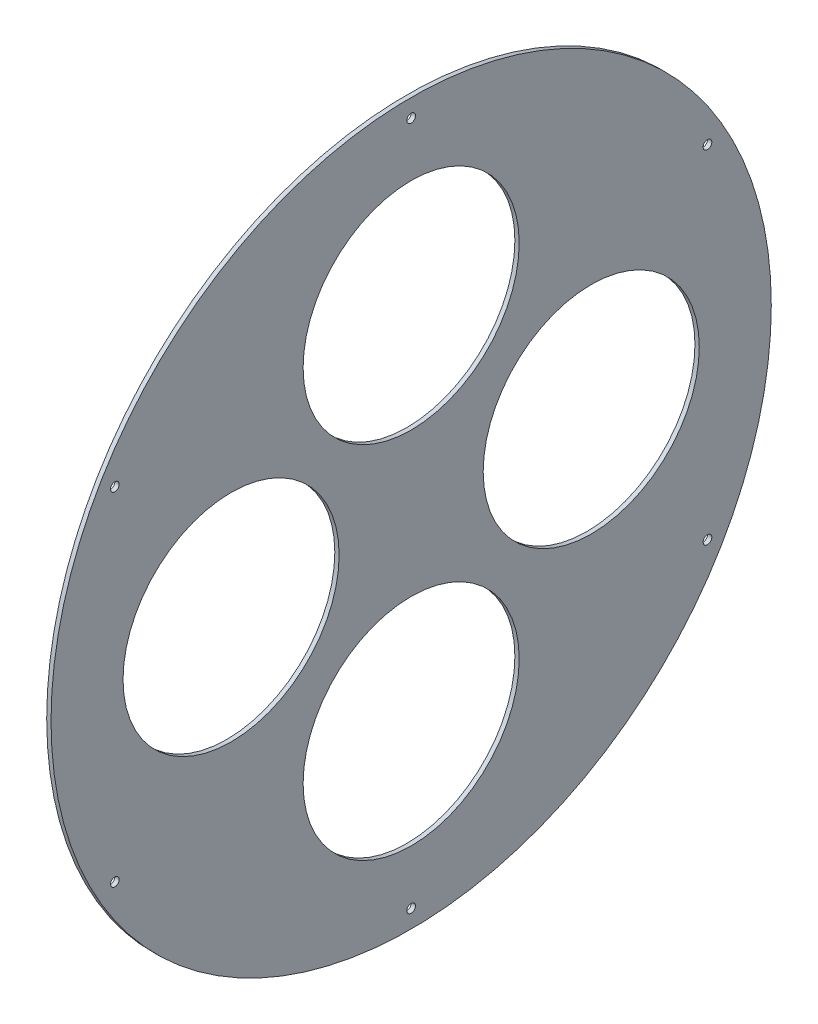
from build123d import *

# Parameters (mm, degrees)
SKETCH1_R           = 250
BOSS_EXTRUDE1_DEPTH = 3
SKETCH2_R           = 75
CUT_EXTRUDE1_DEPTH  = 10
CIRPATTERN1_COUNT   = 4
SKETCH3_R           = 3
CUT_EXTRUDE2_DEPTH  = 20
CIRPATTERN2_COUNT   = 6


with BuildPart() as part:
    # Sketch1 → Boss-Extrude1 (new body)
    with BuildSketch(Plane(origin=(0, 0, 0), x_dir=(0, 0, -1), z_dir=(1, 0, 0))):
        Circle(SKETCH1_R)
    extrude(amount=BOSS_EXTRUDE1_DEPTH)

    # Sketch2 → Cut-Extrude1 (cut)
    with BuildSketch(Plane(origin=(3, 0, 0), x_dir=(0, 0, -1), z_dir=(1, 0, 0))):
        with Locations((0, 125)):
            Circle(SKETCH2_R)
    cut_extrude1 = extrude(amount=-CUT_EXTRUDE1_DEPTH, mode=Mode.SUBTRACT)

    # CirPattern1: Cut-Extrude1 ×4 about axis
    cirpattern1_axis = Axis((0, 0, 0), (1, 0, 0))
    for i in range(1, CIRPATTERN1_COUNT):
        add(cut_extrude1.rotate(cirpattern1_axis, i * 360 / CIRPATTERN1_COUNT), mode=Mode.SUBTRACT)

    # Sketch3 → Cut-Extrude2 (cut)
    with BuildSketch(Plane(origin=(3, 0, 0), x_dir=(0, 0, -1), z_dir=(1, 0, 0))):
        with Locations((0, -237.5)):
            Circle(SKETCH3_R)
    cut_extrude2 = extrude(amount=-CUT_EXTRUDE2_DEPTH, mode=Mode.SUBTRACT)

    # CirPattern2: Cut-Extrude2 ×6 about axis
    cirpattern2_axis = Axis((0, 0, 0), (1, 0, 0))
    for i in range(1, CIRPATTERN2_COUNT):
        add(cut_extrude2.rotate(cirpattern2_axis, i * 360 / CIRPATTERN2_COUNT), mode=Mode.SUBTRACT)


solid = part.part
